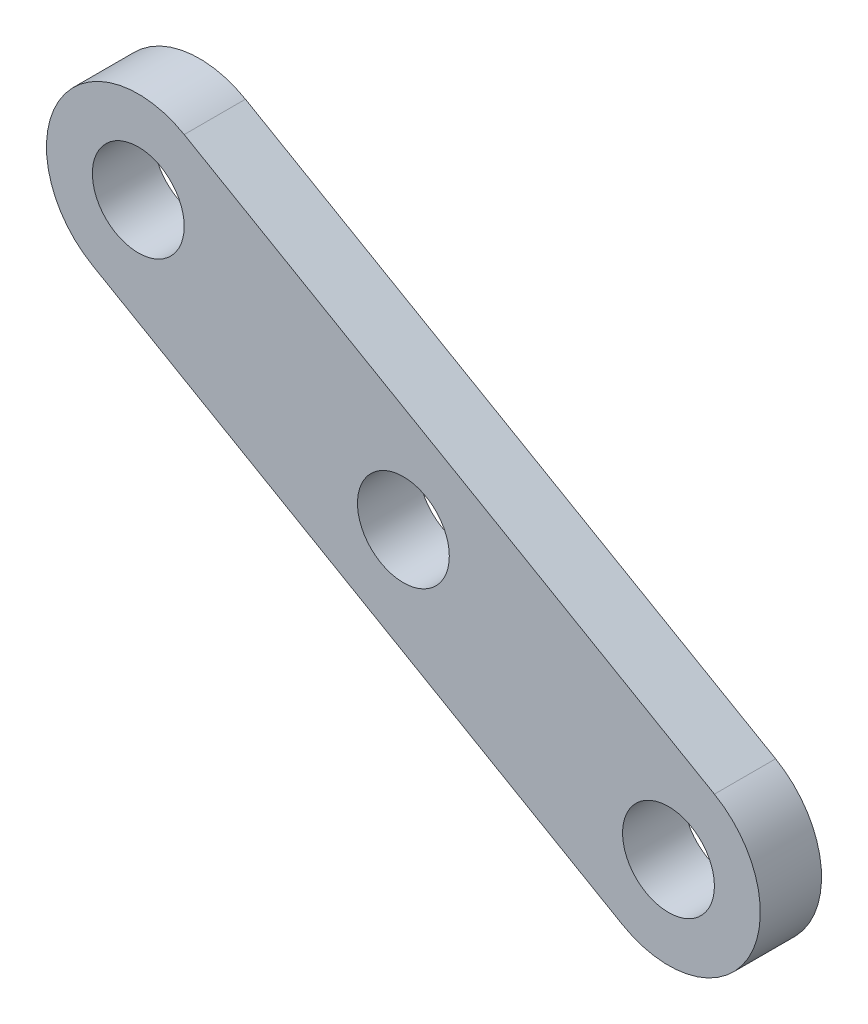
SolidWorks part; units mm, degrees
ref_plane "Front Plane" through (0, 0, 0) normal (0, 0, 1) x (1, 0, 0)
ref_plane "Top Plane" through (0, 0, 0) normal (0, 1, 0) x (1, 0, 0)
ref_plane "Right Plane" through (0, 0, 0) normal (1, 0, 0) x (0, 0, -1)
other "Configuration Table"
sketch "Sketch1" plane through (0, 0, 0) normal (0, 0, 1) x (1, 0, 0)
  line L0 (-8.6603, 5) -> (8.6603, -5) construction
  line L1 (0, 0) -> (50.4196, 0) construction
  line L2 (-10.1603, 2.4019) -> (7.1603, -7.5981)
  line L3 (-7.1603, 7.5981) -> (10.1603, -2.4019)
  circle A0 centre (0, 0) radius 1.5
  arc A1 (-7.1603, 7.5981) -> (-10.1603, 2.4019) centre (-8.6603, 5) ccw
  arc A2 (7.1603, -7.5981) -> (10.1603, -2.4019) centre (8.6603, -5) ccw
  circle A3 centre (8.6603, -5) radius 1.5
  circle A4 centre (-8.6603, 5) radius 1.5
  point P4 (0, 0)
  dimension "D3" = 3
  dimension "D4" = 3
  dimension "D5" = 3
  dimension "D1" = 30
  dimension "D2" = 20
extrude "Boss-Extrude1" add sketch "Sketch1" along normal blind 2
